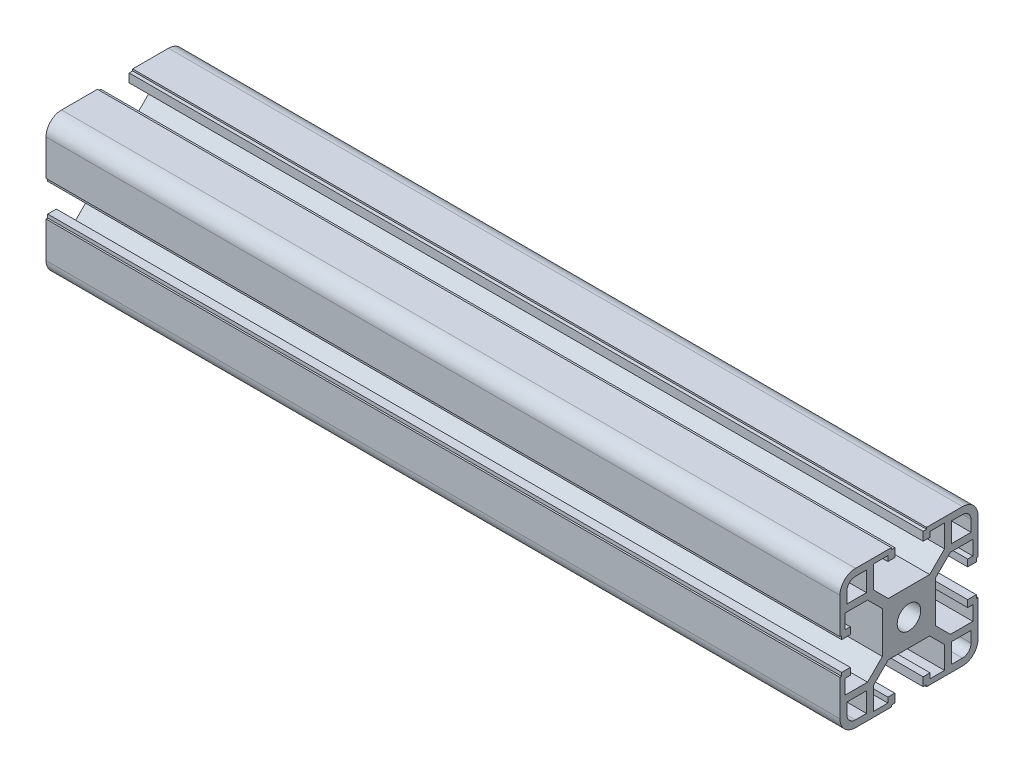
from build123d import *

# Parameters (mm, degrees)
SKETCH1_R                                 = 3.4
ALUMINIUM_PROFILE_40_X_40B_X_R4_5_1_DEPTH = 230


with BuildPart() as part:
    # Sketch1 → Aluminium profile 40 X 40B X R4.5(1) (new body)
    with BuildSketch(Plane.YZ.offset(-984.974958264)):
        with BuildLine():
            Line((-5.1, 20), (-5.1, 19.5))
            Line((-5.1, 19.5), (-4.1, 19.5))
            Line((-4.1, 19.5), (-4.1, 17))
            Line((-4.1, 17), (-6.1, 17))
            Line((-6.1, 17), (-6.1, 18.5))
            Line((-6.1, 18.5), (-10.3, 18.5))
            Line((-10.3, 18.5), (-10.3, 12))
            Line((-10.3, 12), (-6, 7.7))
            Line((-6, 7.7), (6, 7.7))
            Line((6, 7.7), (10.3, 12))
            Line((10.3, 12), (10.3, 18.5))
            Line((10.3, 18.5), (6.1, 18.5))
            Line((6.1, 18.5), (6.1, 17))
            Line((6.1, 17), (4.1, 17))
            Line((4.1, 17), (4.1, 19.5))
            Line((4.1, 19.5), (5.1, 19.5))
            Line((5.1, 19.5), (5.1, 20))
            Line((5.1, 20), (15.5, 20))
            ThreePointArc((15.5, 20), (18.681980515, 18.681980515), (20, 15.5))
            Line((20, 15.5), (20, 5.1))
            Line((20, 5.1), (19.5, 5.1))
            Line((19.5, 5.1), (19.5, 4.1))
            Line((19.5, 4.1), (17, 4.1))
            Line((17, 4.1), (17, 6.1))
            Line((17, 6.1), (18.5, 6.1))
            Line((18.5, 6.1), (18.5, 10.3))
            Line((18.5, 10.3), (12, 10.3))
            Line((12, 10.3), (7.7, 6))
            Line((7.7, 6), (7.7, -6))
            Line((7.7, -6), (12, -10.3))
            Line((12, -10.3), (18.5, -10.3))
            Line((18.5, -10.3), (18.5, -6.1))
            Line((18.5, -6.1), (17, -6.1))
            Line((17, -6.1), (17, -4.1))
            Line((17, -4.1), (19.5, -4.1))
            Line((19.5, -4.1), (19.5, -5.1))
            Line((19.5, -5.1), (20, -5.1))
            Line((20, -5.1), (20, -15.5))
            ThreePointArc((20, -15.5), (18.681980515, -18.681980515), (15.5, -20))
            Line((15.5, -20), (5.1, -20))
            Line((5.1, -20), (5.1, -19.5))
            Line((5.1, -19.5), (4.1, -19.5))
            Line((4.1, -19.5), (4.1, -17))
            Line((4.1, -17), (6.1, -17))
            Line((6.1, -17), (6.1, -18.5))
            Line((6.1, -18.5), (10.3, -18.5))
            Line((10.3, -18.5), (10.3, -12))
            Line((10.3, -12), (6, -7.7))
            Line((6, -7.7), (-6, -7.7))
            Line((-6, -7.7), (-10.3, -12))
            Line((-10.3, -12), (-10.3, -18.5))
            Line((-10.3, -18.5), (-6.1, -18.5))
            Line((-6.1, -18.5), (-6.1, -17))
            Line((-6.1, -17), (-4.1, -17))
            Line((-4.1, -17), (-4.1, -19.5))
            Line((-4.1, -19.5), (-5.1, -19.5))
            Line((-5.1, -19.5), (-5.1, -20))
            Line((-5.1, -20), (-15.5, -20))
            ThreePointArc((-15.5, -20), (-18.681980515, -18.681980515), (-20, -15.5))
            Line((-20, -15.5), (-20, -5.1))
            Line((-20, -5.1), (-19.5, -5.1))
            Line((-19.5, -5.1), (-19.5, -4.1))
            Line((-19.5, -4.1), (-17, -4.1))
            Line((-17, -4.1), (-17, -6.1))
            Line((-17, -6.1), (-18.5, -6.1))
            Line((-18.5, -6.1), (-18.5, -10.3))
            Line((-18.5, -10.3), (-12, -10.3))
            Line((-12, -10.3), (-7.7, -6))
            Line((-7.7, -6), (-7.7, 6))
            Line((-7.7, 6), (-12, 10.3))
            Line((-12, 10.3), (-18.5, 10.3))
            Line((-18.5, 10.3), (-18.5, 6.1))
            Line((-18.5, 6.1), (-17, 6.1))
            Line((-17, 6.1), (-17, 4.1))
            Line((-17, 4.1), (-19.5, 4.1))
            Line((-19.5, 4.1), (-19.5, 5.1))
            Line((-19.5, 5.1), (-20, 5.1))
            Line((-20, 5.1), (-20, 15.5))
            ThreePointArc((-20, 15.5), (-18.681980515, 18.681980515), (-15.5, 20))
            Line((-15.5, 20), (-5.1, 20))
        make_face()
        Circle(SKETCH1_R, mode=Mode.SUBTRACT)
        with BuildLine():
            Line((12.3, 18), (15.5, 18))
            ThreePointArc((15.5, 18), (17.267766953, 17.267766953), (18, 15.5))
            Line((18, 15.5), (18, 12.3))
            Line((18, 12.3), (12.3, 12.3))
            Line((12.3, 12.3), (12.3, 18))
        make_face(mode=Mode.SUBTRACT)
        with BuildLine():
            Line((-15.5, 18), (-12.3, 18))
            Line((-12.3, 18), (-12.3, 12.3))
            Line((-12.3, 12.3), (-18, 12.3))
            Line((-18, 12.3), (-18, 15.5))
            ThreePointArc((-18, 15.5), (-17.267766953, 17.267766953), (-15.5, 18))
        make_face(mode=Mode.SUBTRACT)
        with BuildLine():
            Line((-18, -12.3), (-12.3, -12.3))
            Line((-12.3, -12.3), (-12.3, -18))
            Line((-12.3, -18), (-15.5, -18))
            ThreePointArc((-15.5, -18), (-17.267766953, -17.267766953), (-18, -15.5))
            Line((-18, -15.5), (-18, -12.3))
        make_face(mode=Mode.SUBTRACT)
        with BuildLine():
            Line((12.3, -12.3), (18, -12.3))
            Line((18, -12.3), (18, -15.5))
            ThreePointArc((18, -15.5), (17.267766953, -17.267766953), (15.5, -18))
            Line((15.5, -18), (12.3, -18))
            Line((12.3, -18), (12.3, -12.3))
        make_face(mode=Mode.SUBTRACT)
    extrude(amount=ALUMINIUM_PROFILE_40_X_40B_X_R4_5_1_DEPTH)


solid = part.part
